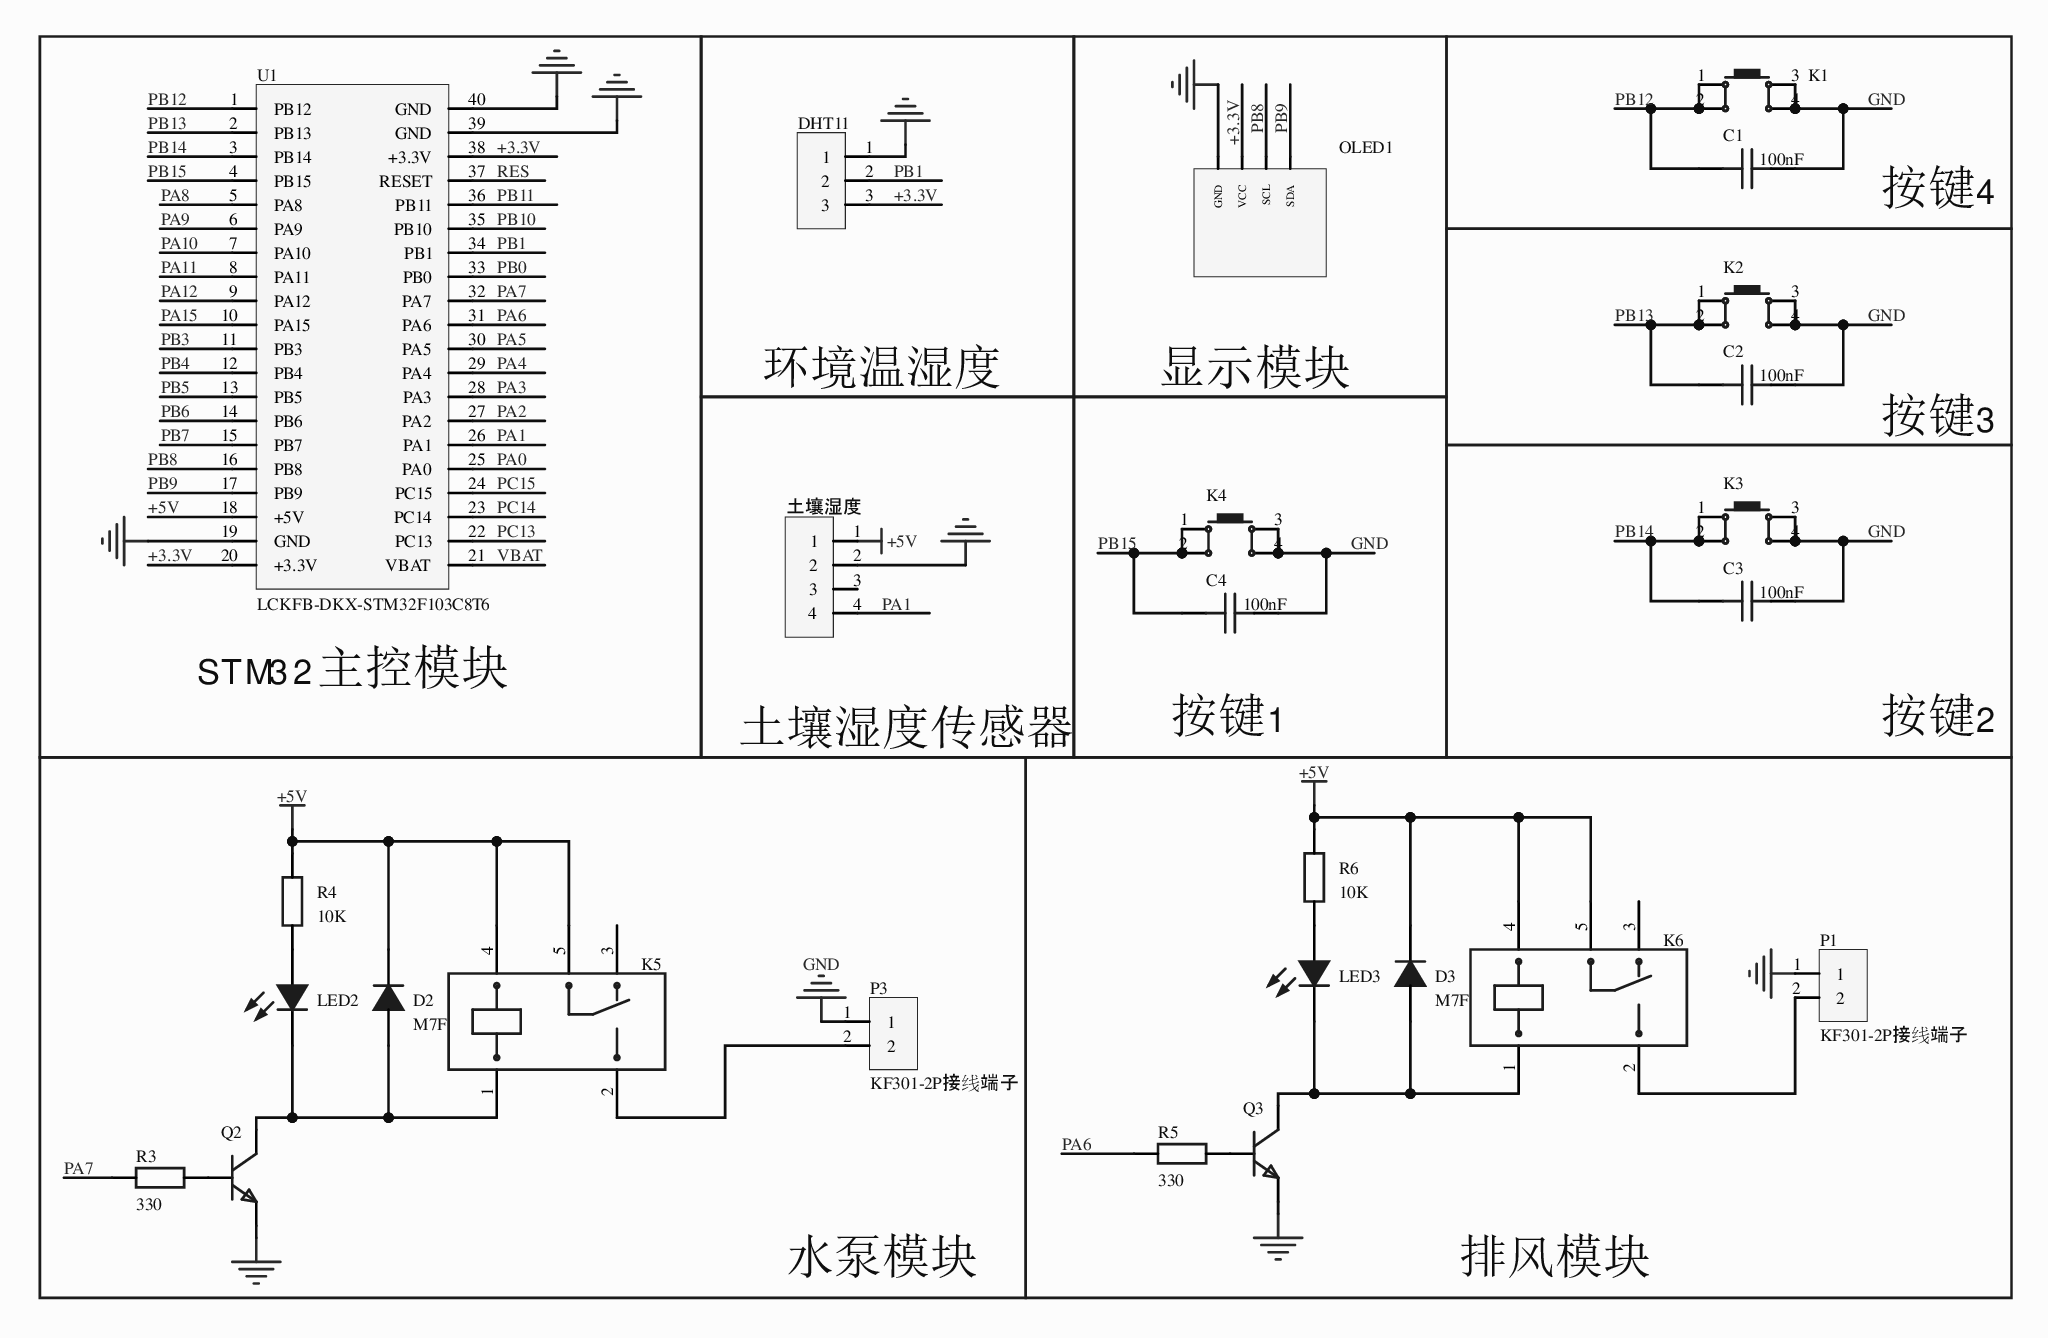
[diagram p0: MISC51528-3.schdoc]
# Altium project MISC51528-2.PrjPcb
1 sheet, 26 parts. Net scope: global (net labels, ports and power ports of the same name join across sheets).
Board file: MISC51528.pcbdoc

## Sheet MISC51528-3.schdoc
size 297 x 209 mm; Version: V1.0; @Project Name: MISC51528; @Update Date: 2026-09-23; @Create Date: 2026-09-23; @Board Name: MISC51528; @Create Time: 19:56:58; @Page Count: 1; @Page No: 1; @Schematic Name: MISC51528; @Update Time: 19:56:58; Size: A4

### Parts
C1  100nF  [C0805]
C2  100nF  [C0805]
C3  100nF  [C0805]
C4  100nF  [C0805]
D2  M7F  [SMAF_L3.5-W2.6-LS4.7-RD]
D3  M7F  [SMAF_L3.5-W2.6-LS4.7-RD]
DHT11  (no value)  [HDR-TH_3P-P2.54-V-M]
K1  (no value)  [SW-SMD_4P-L6.0-W6.0-P4.50-LS9.0-2]
K2  (no value)  [SW-SMD_4P-L6.0-W6.0-P4.50-LS9.0-2]
K3  (no value)  [SW-SMD_4P-L6.0-W6.0-P4.50-LS9.0-2]
K4  (no value)  [SW-SMD_4P-L6.0-W6.0-P4.50-LS9.0-2]
K5  SRD-DC5V-SL-C  [RELAY-TH_SRD-DCXXV-SL-C]  (value not drawn)
K6  SRD-DC5V-SL-C  [RELAY-TH_SRD-DCXXV-SL-C]  (value not drawn)
LED2  MS-PTV1608NWAF-B02  [LED0805-RD_BLUE]  (value not drawn)
LED3  MS-PTV1608NWAF-B02  [LED0805-RD_BLUE]  (value not drawn)
OLED1  (no value)  [0.96OLED_4P]
P1  KF301-2P接线端子  [CONN-TH_XY301V-A-5.0-2P]
P3  KF301-2P接线端子  [CONN-TH_XY301V-A-5.0-2P]
Q2  (no value)  [S8050_SOT-23]
Q3  (no value)  [S8050_SOT-23]
R3  330  [R0805]
R4  10K  [R0805]
R5  330  [R0805]
R6  10K  [R0805]
U1  LCKFB-DKX-STM32F103C8T6  [CONN-TH_L53.3-W22.9_STM32F103C8T6-CARD]
土壤湿度  (no value)  [HDR-TH_4P-P2.54-V-M]

### Blocks framed on the sheet
STM32主控模块: U1
环境温湿度: DHT11
显示模块: OLED1
按键4: C1 K1
按键3: C2 K2
土壤湿度传感器: 土壤湿度
按键1: C4 K4
按键2: C3 K3
水泵模块: D2 K5 LED2 P3 Q2 R3 R4
排风模块: D3 K6 LED3 P1 Q3 R5 R6

### Nets
+5V: D2.1(C) D3.1(C) K5.4 K5.5 K6.4 K6.5 R4.2 R6.2 U1.18(+5V) 土壤湿度.1
GND: C1.2 C2.2 C3.2 C4.2 DHT11.1 K1.3 K1.4 K2.3 K2.4 K3.3 K3.4 K4.3 K4.4 OLED1.1(GND) P1.1 P3.1 Q2.2 Q3.2 U1.19(GND) U1.39(GND) U1.40(GND) 土壤湿度.2
+3.3V: DHT11.3 OLED1.2(VCC) U1.20(+3.3V) U1.38(+3.3V)
PA0: U1.25(PA0)
PA1: U1.26(PA1) 土壤湿度.4
PA2: U1.27(PA2)
PA3: U1.28(PA3)
PA4: U1.29(PA4)
PA5: U1.30(PA5)
PA6: R5.2 U1.31(PA6)
PA7: R3.2 U1.32(PA7)
PA8: U1.5(PA8)
PA9: U1.6(PA9)
PA10: U1.7(PA10)
PA11: U1.8(PA11)
PA12: U1.9(PA12)
PA15: U1.10(PA15)
PB0: U1.33(PB0)
PB1: DHT11.2 U1.34(PB1)
PB3: U1.11(PB3)
PB4: U1.12(PB4)
PB5: U1.13(PB5)
PB6: U1.14(PB6)
PB7: U1.15(PB7)
PB8: OLED1.3(SCL) U1.16(PB8)
PB9: OLED1.4(SDA) U1.17(PB9)
PB10: U1.35(PB10)
PB11: U1.36(PB11)
PB12: C1.1 K1.1 K1.2 U1.1(PB12)
PB13: C2.1 K2.1 K2.2 U1.2(PB13)
PB14: C3.1 K3.1 K3.2 U1.3(PB14)
PB15: C4.1 K4.1 K4.2 U1.4(PB15)
PC13: U1.22(PC13)
PC14: U1.23(PC14)
PC15: U1.24(PC15)
RES: U1.37(RESET)
VBAT: U1.21(VBAT)
NetD2_2: D2.2(A) K5.1 LED2.1(-) Q2.3
NetD3_2: D3.2(A) K6.1 LED3.1(-) Q3.3
NetK5_2: K5.2 P3.2
NetK6_2: K6.2 P1.2
NetLED2_2: LED2.2(+) R4.1
NetLED3_2: LED3.2(+) R6.1
NetQ2_1: Q2.1 R3.1
NetQ3_1: Q3.1 R5.1

Not connected (* = marked no-connect by the designer): K5 3*; K6 3*; 土壤湿度 3*

### Library data of the parts
C1-C4 = CC0603KRX7R5BB104: 容值:100nF;精度:±10%;额定电压:6.3V;材质(温度系数):X7R;; Manufacturer: YAGEO(国巨); 3D Model: ac125912035d415993ca9572d50418b1; 3D Model Transform: 62.992,31.496,0,0,0,0,0,0,0; Tolerance: ±10%; Voltage Rated: 6.3V; Temperature Coefficient: X7R; AddInBom: yes; ModelName: C0603_L1.6-W0.8-H0.8; Symbol: CC0603KRX7R5BB104; Device: CC0603KRX7R5BB104; LCSC Part Name: 100nF ±10% 6.3V; Supplier Part: C5445386; Manufacturer Part: CC0603KRX7R5BB104; Supplier Footprint: 0603; Datasheet: https://atta.szlcsc.com/upload/public/pdf/source/20230424/E18B5086BA02F13791E1DFCA214F4995.pdf; Supplier: LCSC; Value: 100nF; ConvertToPcb: yes; FootprintName: C0805
D2 D3 = M7F_C22368801: 正向压降(Vf):1.1V@1A;直流反向耐压(Vr):1kV;整流电流:1A;; Manufacturer: Wild Goose(威谷); 3D Model: 4caf566195a049cf809ac17c4d641932; 3D Model Transform: 183.0705,102.362,0,0,0,0,0,0,0; Voltage - DC Reverse(Vr): 1kV; Current - Rectified: 1A; Reverse Leakage Current (Ir): 5uA@1kV; Non-Repetitive Peak Forward Surge Current: 30A; AddInBom: yes; ModelName: SMAF_L3.5-W2.6-LS4.7-RD-1; Symbol: M7F_C22368801; Device: M7F_C22368801; LCSC Part Name: M7F; Supplier Part: C22368801; Manufacturer Part: M7F; Supplier Footprint: SMAF; JLCPCB Part Class: 扩展库; Datasheet: https://item.szlcsc.com/datasheet/M7F/23847113.html; Supplier: LCSC; Voltage - Forward(Vf@If): 1.1V@1A; ConvertToPcb: yes; FootprintName: SMAF_L3.5-W2.6-LS4.7-RD
DHT11 = HDR-M_2.54_1x3P: 3D Model: bb473b6d38ff42a99216a4fcdbdcc4cb0819f05c4eef4c71ace90d822a990e87; 3D Model Transform: 300.03877,100,0,0,0,0,0,0,-118.11; AddInBom: yes; ModelName: HDR-TH_3P-P2.54-M-LI-1X3P; Symbol: HDR-M_2.54_1x3P; Device: HDR-M_2.54_1x3P; Supplier Part: C2937625; Supplier Footprint: 插件; FootprintName: HDR-TH_3P-P2.54-V-M; ConvertToPcb: yes
K1-K4 = Key_SMD_6x6x6.5: Symbol: 轻触按键; 3D Model: fbf4ceca6c4742d48614ab6a891ef981; 3D Model Transform: 330.708,251.968,0,0,0,0,0,-0.005,0; ConvertToPcb: yes; ModelName: SW-SMD_4P-L6.0-W6.0-P4.50-LS11.0; Device: Key_SMD_6x6x6.5; Supplier Footprint: SMD; AddInBom: yes; FootprintName: SW-SMD_4P-L6.0-W6.0-P4.50-LS9.0-2
K5 K6 = SRD-DC5V-SL-C: 触点形式:-;; 3D Model: d0eda9b8bf8746d18ae810ab88dc78e7; 3D Model Transform: 755.904,622.4397,0,0,0,0,34.882,0,-118.11; AddInBom: yes; ModelName: RELAY-TH_L19.2-W15.6-H15.8; Symbol: SRD-DC5V-SL-C; Device: SRD-DC5V-SL-C; LCSC Part Name: SRD-DC5V-SL-C; Supplier Part: C688865; Manufacturer Part: SRD-DC5V-SL-C; Supplier Footprint: 插件; JLCPCB Part Class: 扩展库; Supplier: LCSC; Contact Form: -; Coil Type: -; ConvertToPcb: yes; FootprintName: RELAY-TH_SRD-DCXXV-SL-C
LED2 LED3 = MS-PTV1608NWAF-B02: 3D Model: 1f0d29a91be547639d425604e9b96ebb; 3D Model Transform: 63.7794,32.283,0,0,0,0,0,0,0; AddInBom: yes; ModelName: LED0603-RD; Symbol: MS-PTV1608NWAF-B02; Device: MS-PTV1608NWAF-B02; LCSC Part Name: MS-PTV1608NWAF-B02; Supplier Part: C9900092855; Manufacturer Part: MS-PTV1608NWAF-B02; Supplier Footprint: LED0603; JLCPCB Part Class: 扩展库; Supplier: LCSC; ConvertToPcb: yes; FootprintName: LED0805-RD_BLUE
OLED1 = 0.96OLED模块_4P: 3D Model: 79c000fdb68d45a296c2e9bedf4f9055; 3D Model Transform: 1393.69792,1318.895,0,0,0,0,0,-560.079,-137.795; ConvertToPcb: yes; Symbol: 0.96OLED模块_4P; Device: 0.96OLED模块_4P; Supplier Footprint: 插件; AddInBom: yes; FootprintName: 0.96OLED_4P; ModelName: 0.96OLED_4P
P1 P3 = KF301-2P接线端子: 3D Model: ef7ead88b0f2448d904975b26718870f; 3D Model Transform: 417.322,299.212,0,0,0,0,11.811,-7.835,-157.48; AddInBom: yes; Symbol: KF301-2P接线端子; Device: KF301-2P接线端子; LCSC Part Name: KF301-2P接线端子; Supplier Part: C9900016950; Manufacturer Part: KF301-2P接线端子; Supplier Footprint: CK301-2P; JLCPCB Part Class: 扩展库; Supplier: LCSC; ConvertToPcb: yes; FootprintName: CONN-TH_XY301V-A-5.0-2P; ModelName: CONN-TH_XY301V-A-5.0-2P
Q2 Q3 = S8050_SOT_NPN: Symbol: NPN; 3D Model: c62791f0466c4ae2a892c056b845b0ca; 3D Model Transform: 98.6,114.12,41.29,180,0,0,0,0,-3; ConvertToPcb: yes; ModelName: SOT-23-3P_L2.9-W1.3-H1.0-LS2.4-P0.95; Device: S8050_SOT_NPN; Supplier Footprint: SOT-23; AddInBom: yes; FootprintName: S8050_SOT-23
R3-R6 = Res_0603: Symbol: 电阻; 3D Model: fc143cca1e79419f9cd78b61e9279f08; 3D Model Transform: 31.8897,63.7794,0,90,0,0,0,0,0; ConvertToPcb: yes; ModelName: R0603; Device: Res_0603; Supplier Footprint: 0603; AddInBom: yes; FootprintName: R0805
  R3 R5: Value: 330
  R4 R6: Value: 10K
U1 = LCKFB-DKX-STM32F103C8T6: Manufacturer: 立创开发板; AddInBom: yes; Symbol: LCKFB-DKX-STM32F103C8T6; Device: LCKFB-DKX-STM32F103C8T6; LCSC Part Name: 立创·地阔星-STM32F103C8T6开发板; Supplier Part: C22396880; Manufacturer Part: LCKFB-DKX-STM32F103C8T6; Supplier Footprint: -; JLCPCB Part Class: 扩展库; Datasheet: https://item.szlcsc.com/datasheet/LCKFB-DKX-STM32F103C8T6/24005615.html; Supplier: LCSC; ConvertToPcb: yes; FootprintName: CONN-TH_L53.3-W22.9_STM32F103C8T6-CARD
土壤湿度 = HDR-M_2.54_1x4P: Symbol: PZ254V-11-04P; 3D Model: 112f4d05e8d64e99ab9a333894bea4f90819f05c4eef4c71ace90d822a990e87; 3D Model Transform: 399.999,104.7242,0,0,0,0,0,0,-118.11; ConvertToPcb: yes; ModelName: HDR-TH_4P-P2.54-M-LI-1X4P; Device: HDR-M_2.54_1x4P; Supplier Part: C492403; Supplier Footprint: 插件; FootprintName: HDR-TH_4P-P2.54-V-M; AddInBom: yes